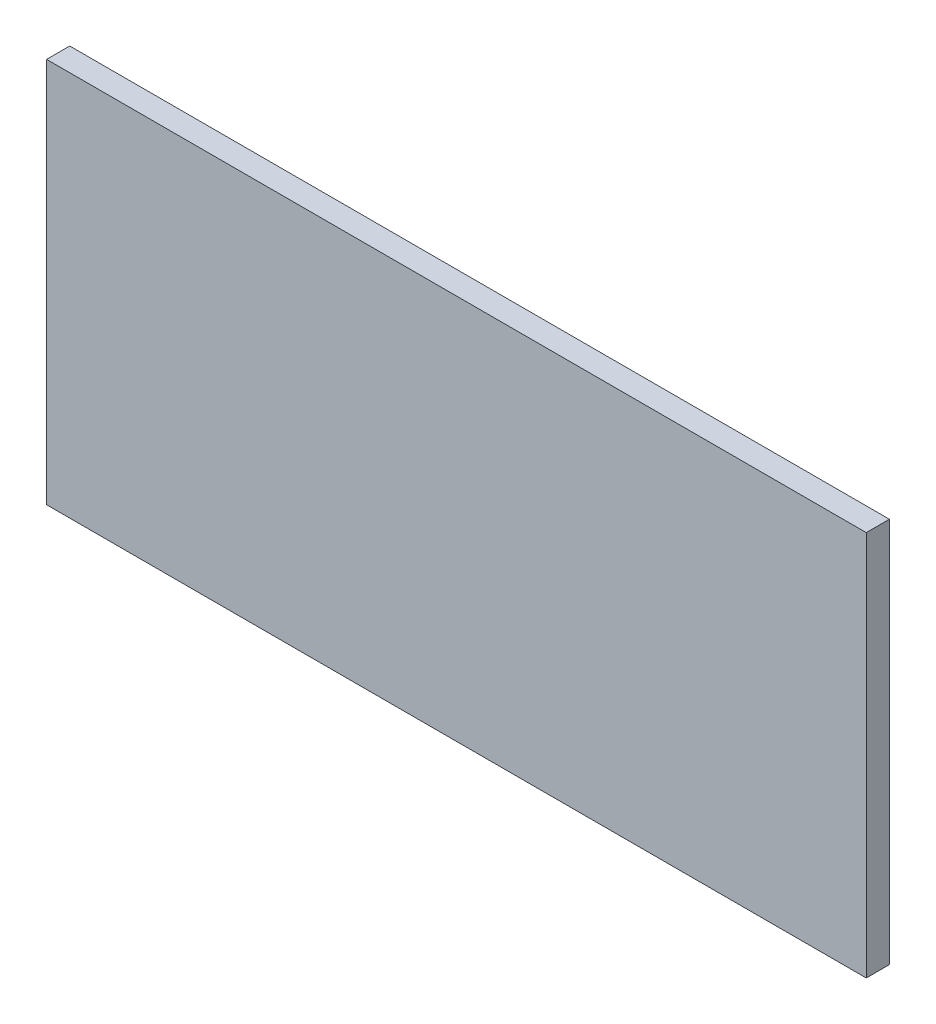
SolidWorks part; units mm, degrees
material "Q235"
ref_plane "Front Plane" through (0, 0, 0) normal (0, 0, 1) x (1, 0, 0)
ref_plane "Top Plane" through (0, 0, 0) normal (0, 1, 0) x (1, 0, 0)
ref_plane "Right Plane" through (0, 0, 0) normal (1, 0, 0) x (0, 0, -1)
sketch "Sketch1" plane through (0, 0, 0) normal (0, 0, 1) x (1, 0, 0)
  line L1 (0, 0) -> (425, 0)
  line L2 (0, 0) -> (0, 200)
  line L3 (0, 200) -> (425, 200)
  line L4 (425, 0) -> (425, 200)
  dimension "D1" = 425
  dimension "D2" = 200
extrude "Boss-Extrude1" add sketch "Sketch1" along normal blind 12
